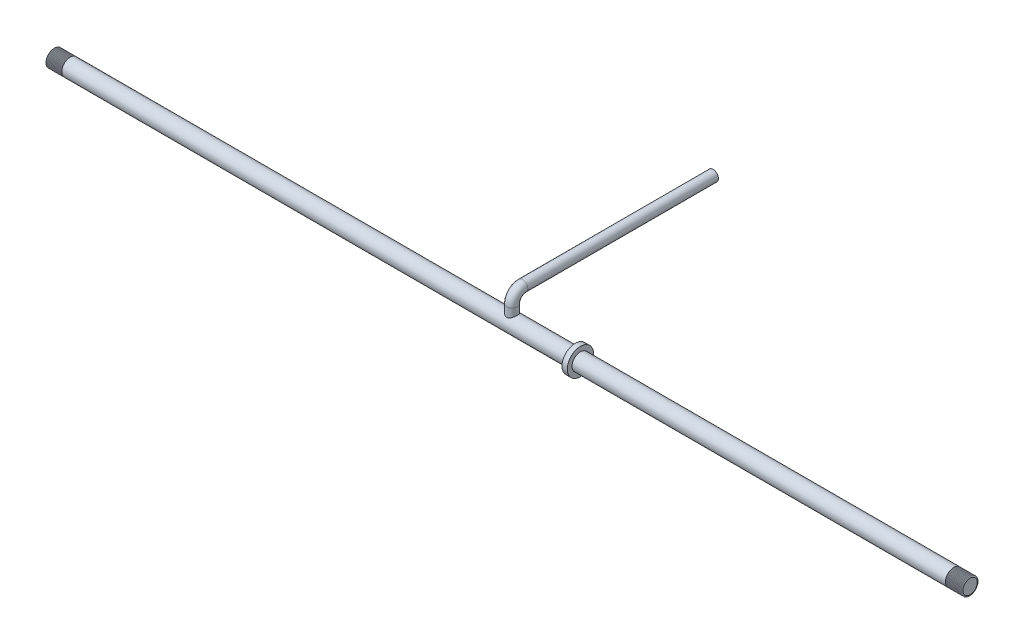
SolidWorks part; units mm, degrees
ref_plane "前视基准面" through (0, 0, 0) normal (0, 0, 1) x (1, 0, 0)
ref_plane "上视基准面" through (0, 0, 0) normal (0, 1, 0) x (1, 0, 0)
ref_plane "右视基准面" through (0, 0, 0) normal (1, 0, 0) x (0, 0, -1)
sketch "草图2" plane through (0, 0, 0) normal (1, 0, 0) x (0, 0, -1)
  line L0 (0, 0) -> (0, 15)
  line L1 (10, 25) -> (191, 25)
  arc A0 (10, 25) -> (0, 15) centre (10, 15) ccw
  dimension "D1" = 10
sketch "草图3" plane through (0, 0, 0) normal (0, 1, 0) x (1, 0, 0)
  circle A0 centre (0, 0) radius 5
sweep "扫描1" add profiles "草图3" path "草图2"
sketch "草图4" plane through (0, 0, 0) normal (1, 0, 0) x (0, 0, -1)
  circle A0 centre (0, 0) radius 8
extrude "凸台-拉伸2" add sketch "草图4" along normal mid plane 870 separate body
sketch "草图7" plane through (0, 0, 0) normal (0, 1, 0) x (1, 0, 0)
  line L0 (442.1611, 0) -> (411.9692, 0) construction
  line L1 (420, 8) -> (420.5, 8)
  line L2 (420.5, 8) -> (420, 6.8)
  line L4 (420, 6.8) -> (419.5, 8)
  line L6 (419.5, 8) -> (420, 8)
  dimension "D1" = 0.5
  dimension "D2" = 1.2
revolve "切除-旋转1" cut sketch "草图7" angle 360 about L0
pattern_linear "阵列(线性)1" count 16 spacing 1 along (1, 0, 0) of "切除-旋转1"
mirror "镜向2" about plane through (0, 0, 0) normal (1, 0, 0) of "阵列(线性)1", "切除-旋转1"
ref_plane "基准面1" through (60, 0, 0) normal (1, 0, 0) x (0, 0, -1)
sketch "草图8" plane through (60, 0, 0) normal (1, 0, 0) x (0, 0, -1)
  circle A0 centre (0, 0) radius 12.5
extrude "凸台-拉伸3" add sketch "草图8" along normal blind 5
